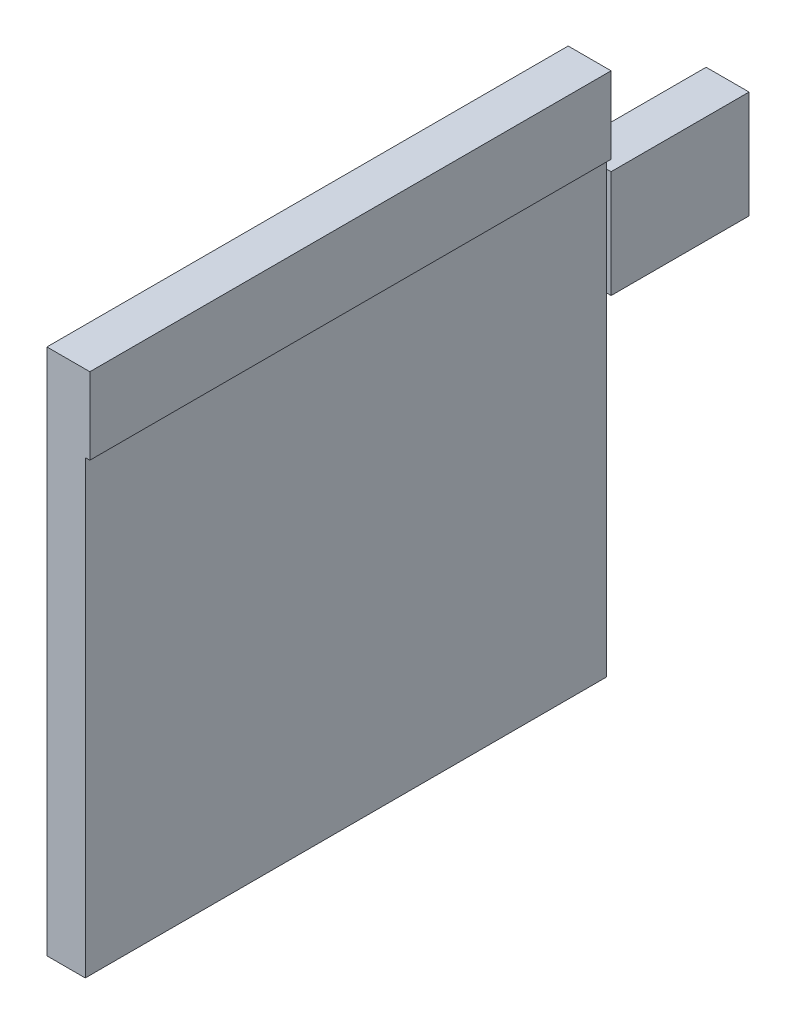
from build123d import *

# Parameters (mm, degrees)
EXTRUDE_1_DEPTH = 85
SKETCH_4_W      = 14
SKETCH_4_H      = 35
EXTRUDE_2_DEPTH = 45


with BuildPart() as part:
    # 草图1 → 凸台-拉伸1 (new, symmetric)
    with BuildSketch(Plane.XY):
        Polygon((0, 0), (0, 172), (14, 172), (14, 147), (12.5, 147), (12.5, 0), align=None)
    extrude(amount=EXTRUDE_1_DEPTH, both=True)

    # 草图4 → 凸台-拉伸2 (add)
    with BuildSketch(Plane(origin=(0, 0, -85), x_dir=(-1, 0, 0), z_dir=(0, 0, -1))):
        with Locations((-7, 126)):
            Rectangle(SKETCH_4_W, SKETCH_4_H)
    extrude(amount=EXTRUDE_2_DEPTH)


solid = part.part
